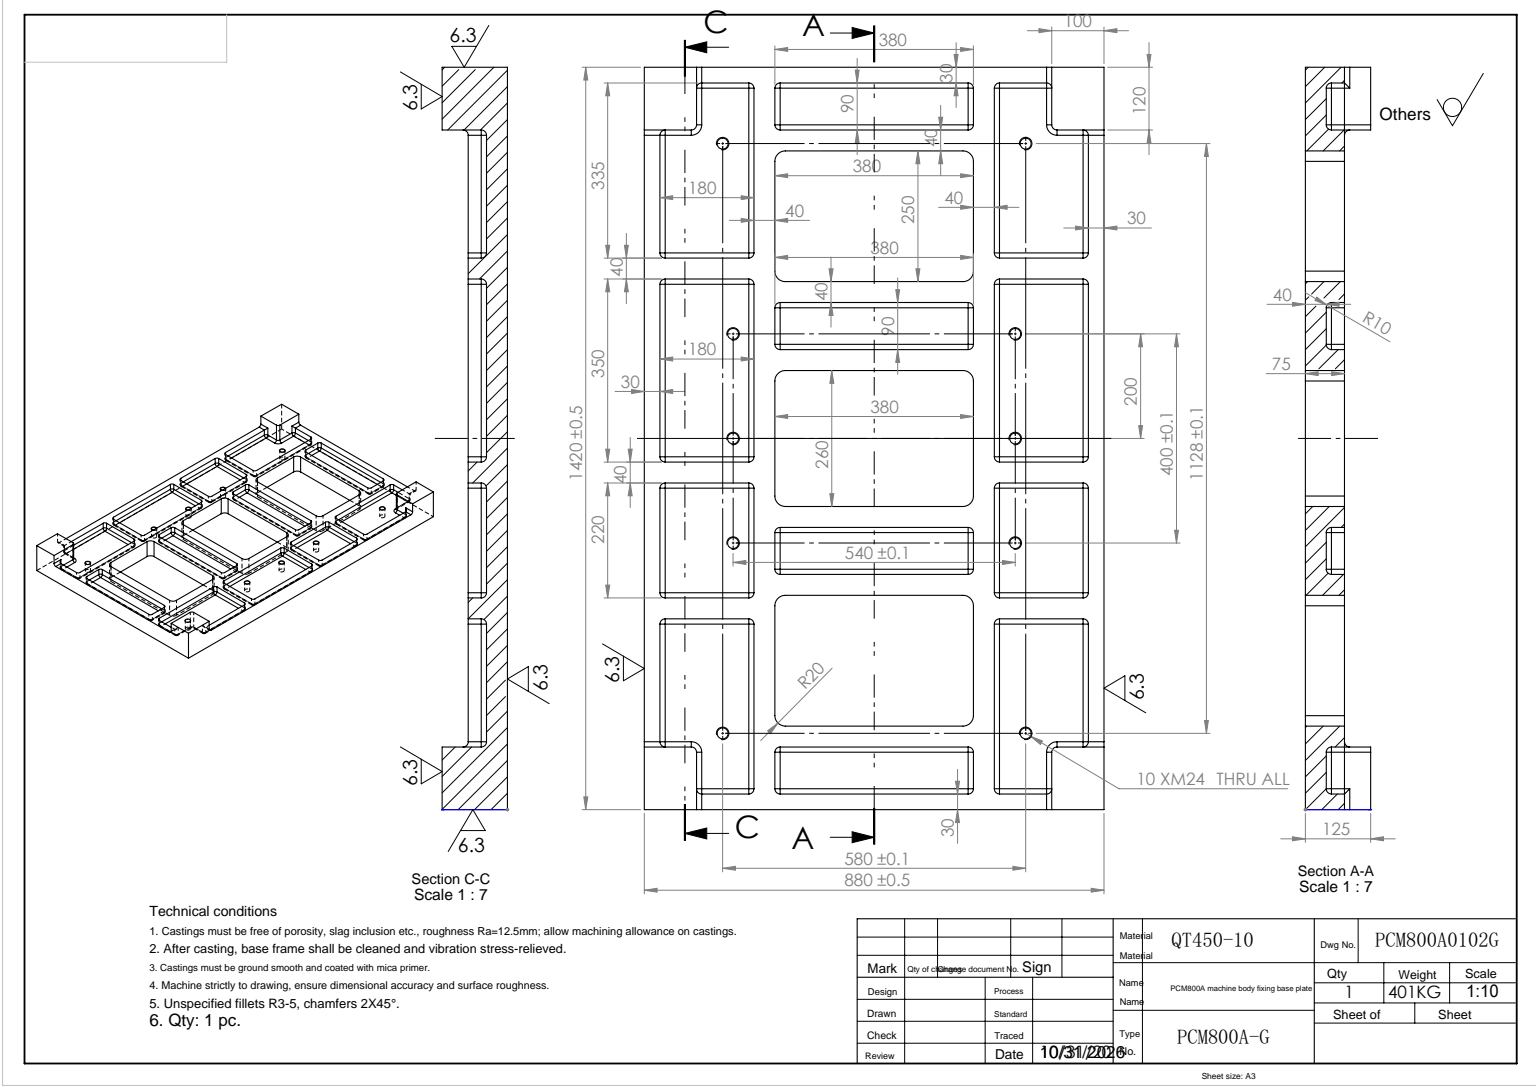
from build123d import *

# Parameters (mm, degrees)
SKETCH_1_W                  = 880
SKETCH_1_H                  = 75
EXTRUDE_1_DEPTH             = 1420
SKETCH_3_W                  = 380
SKETCH_3_H                  = 260
SKETCH_3_H_2                = 250
CUT_EXTRUDE_1_DEPTH         = 1673.251476304
SKETCH_4_W                  = 180
SKETCH_4_H                  = 335
SKETCH_4_H_2                = 350
SKETCH_4_H_3                = 220
SKETCH_4_W_2                = 380
SKETCH_4_H_4                = 90
CUT_EXTRUDE_2_DEPTH         = 35
FILLET_11_R                 = 20
FILLET_1_R                  = 10
HOLE_WIZARD_M24_1_D         = 21
PATTERN_LINEAR_2_COUNT      = 2
PATTERN_LINEAR_2_PITCH      = 580
PATTERN_LINEAR_2_COUNT_DIR2 = 2
PATTERN_LINEAR_2_PITCH_DIR2 = 1128
HOLE_WIZARD_M24_2_D         = 21
PATTERN_LINEAR_3_COUNT      = 2
PATTERN_LINEAR_3_PITCH      = 540
PATTERN_LINEAR_3_COUNT_DIR2 = 3
PATTERN_LINEAR_3_PITCH_DIR2 = 200
SKETCH_9_W                  = 100
SKETCH_9_H                  = 120
EXTRUDE_1_2_DEPTH           = 85
FILLET_12_R                 = 10


with BuildPart() as part:
    # 草图1 → Extrude 1 (new body)
    with BuildSketch(Plane.XY):
        with Locations((440, 37.5)):
            Rectangle(SKETCH_1_W, SKETCH_1_H)
    extrude(amount=EXTRUDE_1_DEPTH)

    # 草图3 → 切除-拉伸1 (cut, through all)
    with BuildSketch(Plane.XZ):
        with Locations((440, 710)):
            Rectangle(SKETCH_3_W, SKETCH_3_H)
        with Locations((440, 1135)):
            Rectangle(SKETCH_3_W, SKETCH_3_H_2)
        with Locations((440, 285)):
            Rectangle(SKETCH_3_W, SKETCH_3_H_2)
    extrude(amount=-CUT_EXTRUDE_1_DEPTH, mode=Mode.SUBTRACT)

    # 草图4 → 切除-拉伸2 (cut)
    with BuildSketch(Plane.XZ.offset(-75)):
        with Locations((760, 1222.5)):
            Rectangle(SKETCH_4_W, SKETCH_4_H)
        with Locations((120, 840)):
            Rectangle(SKETCH_4_W, SKETCH_4_H_2)
        with Locations((760, 840)):
            Rectangle(SKETCH_4_W, SKETCH_4_H_2)
        with Locations((760, 515)):
            Rectangle(SKETCH_4_W, SKETCH_4_H_3)
        with Locations((760, 197.5)):
            Rectangle(SKETCH_4_W, SKETCH_4_H)
        with Locations((120, 1222.5)):
            Rectangle(SKETCH_4_W, SKETCH_4_H)
        with Locations((120, 515)):
            Rectangle(SKETCH_4_W, SKETCH_4_H_3)
        with Locations((120, 197.5)):
            Rectangle(SKETCH_4_W, SKETCH_4_H)
        with Locations((440, 495)):
            Rectangle(SKETCH_4_W_2, SKETCH_4_H_4)
        with Locations((440, 925)):
            Rectangle(SKETCH_4_W_2, SKETCH_4_H_4)
        with Locations((440, 1345)):
            Rectangle(SKETCH_4_W_2, SKETCH_4_H_4)
        with Locations((440, 75)):
            Rectangle(SKETCH_4_W_2, SKETCH_4_H_4)
    extrude(amount=CUT_EXTRUDE_2_DEPTH, mode=Mode.SUBTRACT)

    # 圆角11
    fillet_11_edges = [part.edges().sort_by_distance(p)[0] for p in [
        (250, 37.5, 580),
        (250, 37.5, 840),
        (630, 37.5, 840),
        (630, 37.5, 580),
        (250, 37.5, 1010),
        (250, 37.5, 1260),
        (630, 37.5, 1260),
        (630, 37.5, 1010),
        (250, 37.5, 160),
        (250, 37.5, 410),
        (630, 37.5, 410),
        (630, 37.5, 160),
    ]]
    fillet(fillet_11_edges, radius=FILLET_11_R)

    # 圆角1
    fillet_1_edges = [part.edges().sort_by_distance(p)[0] for p in [
        (30, 57.5, 1015),
        (30, 57.5, 665),
        (210, 57.5, 665),
        (210, 57.5, 1015),
        (30, 40, 840),
        (120, 40, 665),
        (210, 40, 840),
        (120, 40, 1015),
        (210, 57.5, 1390),
        (30, 57.5, 1390),
        (30, 57.5, 1055),
        (210, 57.5, 1055),
        (120, 40, 1390),
        (30, 40, 1222.5),
        (120, 40, 1055),
        (210, 40, 1222.5),
        (30, 57.5, 625),
        (30, 57.5, 405),
        (210, 57.5, 405),
        (210, 57.5, 625),
        (30, 40, 515),
        (120, 40, 405),
        (210, 40, 515),
        (120, 40, 625),
        (30, 57.5, 365),
        (30, 57.5, 30),
        (210, 57.5, 30),
        (210, 57.5, 365),
        (30, 40, 197.5),
        (120, 40, 30),
        (210, 40, 197.5),
        (120, 40, 365),
        (250, 57.5, 970),
        (250, 57.5, 880),
        (630, 57.5, 880),
        (630, 57.5, 970),
        (250, 40, 925),
        (440, 40, 880),
        (630, 40, 925),
        (440, 40, 970),
        (250, 57.5, 540),
        (250, 57.5, 450),
        (630, 57.5, 450),
        (630, 57.5, 540),
        (250, 40, 495),
        (440, 40, 450),
        (630, 40, 495),
        (440, 40, 540),
        (250, 57.5, 1390),
        (250, 57.5, 1300),
        (630, 57.5, 1300),
        (630, 57.5, 1390),
        (250, 40, 1345),
        (440, 40, 1300),
        (630, 40, 1345),
        (440, 40, 1390),
        (250, 57.5, 120),
        (250, 57.5, 30),
        (630, 57.5, 30),
        (630, 57.5, 120),
        (250, 40, 75),
        (440, 40, 30),
        (630, 40, 75),
        (440, 40, 120),
        (850, 57.5, 1055),
        (850, 57.5, 1390),
        (670, 57.5, 1390),
        (670, 57.5, 1055),
        (850, 40, 1222.5),
        (760, 40, 1390),
        (670, 40, 1222.5),
        (760, 40, 1055),
        (850, 57.5, 1015),
        (670, 57.5, 1015),
        (670, 57.5, 665),
        (850, 57.5, 665),
        (760, 40, 1015),
        (670, 40, 840),
        (760, 40, 665),
        (850, 40, 840),
        (850, 57.5, 625),
        (670, 57.5, 625),
        (670, 57.5, 405),
        (850, 57.5, 405),
        (760, 40, 625),
        (670, 40, 515),
        (760, 40, 405),
        (850, 40, 515),
        (850, 57.5, 365),
        (670, 57.5, 365),
        (670, 57.5, 30),
        (850, 57.5, 30),
        (760, 40, 365),
        (670, 40, 197.5),
        (760, 40, 30),
        (850, 40, 197.5),
    ]]
    fillet(fillet_1_edges, radius=FILLET_1_R)

    # M24 螺纹孔1 (through all)
    with Locations(Plane(origin=(150, 40, 146), x_dir=(0, 0, 1), z_dir=(0, 1, 0))):
        with Locations((0, 0)):
            hole_wizard_m24_1 = Hole(HOLE_WIZARD_M24_1_D / 2)

    # 阵列(线性)2: Hole Wizard M24 _1 2 × 2
    with Locations(*[(i * PATTERN_LINEAR_2_PITCH, 0, j * PATTERN_LINEAR_2_PITCH_DIR2) for i in range(PATTERN_LINEAR_2_COUNT) for j in range(PATTERN_LINEAR_2_COUNT_DIR2) if (i, j) != (0, 0)]):
        add(hole_wizard_m24_1, mode=Mode.SUBTRACT)

    # M24 螺纹孔2 (through all)
    with Locations(Plane(origin=(170, 40, 510), x_dir=(0, 0, 1), z_dir=(0, 1, 0))):
        with Locations((0, 0)):
            hole_wizard_m24_2 = Hole(HOLE_WIZARD_M24_2_D / 2)

    # 阵列(线性)3: Hole Wizard M24 _2 2 × 3
    with Locations(*[(i * PATTERN_LINEAR_3_PITCH, 0, j * PATTERN_LINEAR_3_PITCH_DIR2) for i in range(PATTERN_LINEAR_3_COUNT) for j in range(PATTERN_LINEAR_3_COUNT_DIR2) if (i, j) != (0, 0)]):
        add(hole_wizard_m24_2, mode=Mode.SUBTRACT)

    # 草图9 → Extrude 1 2 (add)
    with BuildSketch(Plane(origin=(0, 40, 0), x_dir=(1, 0, 0), z_dir=(0, 1, 0))):
        with Locations((50, -60)):
            Rectangle(SKETCH_9_W, SKETCH_9_H)
        with Locations((830, -60)):
            Rectangle(SKETCH_9_W, SKETCH_9_H)
        with Locations((830, -1360)):
            Rectangle(SKETCH_9_W, SKETCH_9_H)
        with Locations((50, -1360)):
            Rectangle(SKETCH_9_W, SKETCH_9_H)
    extrude(amount=EXTRUDE_1_2_DEPTH)

    # 圆角12
    fillet_12_edges = [part.edges().sort_by_distance(p)[0] for p in [
        (100, 42.928932188, 32.928932188),
        (32.928932188, 42.928932188, 120),
        (15, 75, 120),
        (70, 40, 120),
        (100, 75, 15),
        (100, 82.5, 120),
        (100, 40, 80),
        (30, 62.5, 120),
        (100, 62.5, 30),
        (780, 42.928932188, 32.928932188),
        (847.071067812, 42.928932188, 120),
        (865, 75, 120),
        (780, 82.5, 120),
        (810, 40, 120),
        (780, 75, 15),
        (780, 40, 80),
        (780, 62.5, 30),
        (850, 62.5, 120),
        (780, 42.928932188, 1387.071067812),
        (847.071067812, 42.928932188, 1300),
        (865, 75, 1300),
        (810, 40, 1300),
        (780, 75, 1405),
        (780, 82.5, 1300),
        (780, 40, 1340),
        (850, 62.5, 1300),
        (780, 62.5, 1390),
        (32.928932188, 42.928932188, 1300),
        (100, 42.928932188, 1387.071067812),
        (100, 75, 1405),
        (100, 40, 1340),
        (15, 75, 1300),
        (100, 82.5, 1300),
        (70, 40, 1300),
        (100, 62.5, 1390),
        (30, 62.5, 1300),
    ]]
    fillet(fillet_12_edges, radius=FILLET_12_R)


solid = part.part
